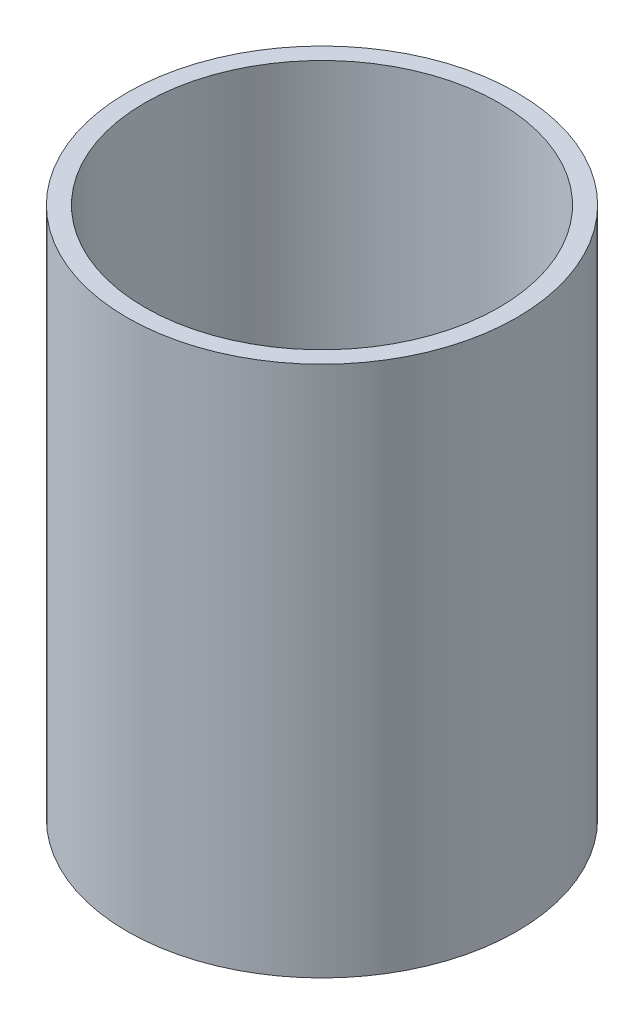
from build123d import *

# Parameters (mm, degrees)
SKETCH1_R           = 110
BOSS_EXTRUDE1_DEPTH = 300
SKETCH3_R           = 100
CUT_EXTRUDE1_DEPTH  = 20
CUT_EXTRUDE2_START  = -270
SKETCH4_R           = 100
CUT_EXTRUDE2_DEPTH  = 270


with BuildPart() as part:
    # Sketch1 → Boss-Extrude1 (new body)
    with BuildSketch(Plane(origin=(0, 0, 0), x_dir=(1, 0, 0), z_dir=(0, 1, 0))):
        with Locations(Location((0, 0, 0), (0, 0, 270))):
            Circle(SKETCH1_R)
    extrude(amount=BOSS_EXTRUDE1_DEPTH)

    # Sketch3 → Cut-Extrude1 (cut)
    with BuildSketch(Plane.XZ):
        with Locations(Location((0, 0, 0), (0, 0, 270))):
            Circle(SKETCH3_R)
    extrude(amount=-CUT_EXTRUDE1_DEPTH, mode=Mode.SUBTRACT)

    # Sketch4 → Cut-Extrude2 (cut)
    with BuildSketch(Plane(origin=(0, 300, 0), x_dir=(1, 0, 0), z_dir=(0, 1, 0)).offset(CUT_EXTRUDE2_START)):
        with Locations(Location((0, 0, 0), (0, 0, 90))):
            Circle(SKETCH4_R)
    extrude(amount=CUT_EXTRUDE2_DEPTH, mode=Mode.SUBTRACT)


solid = part.part
